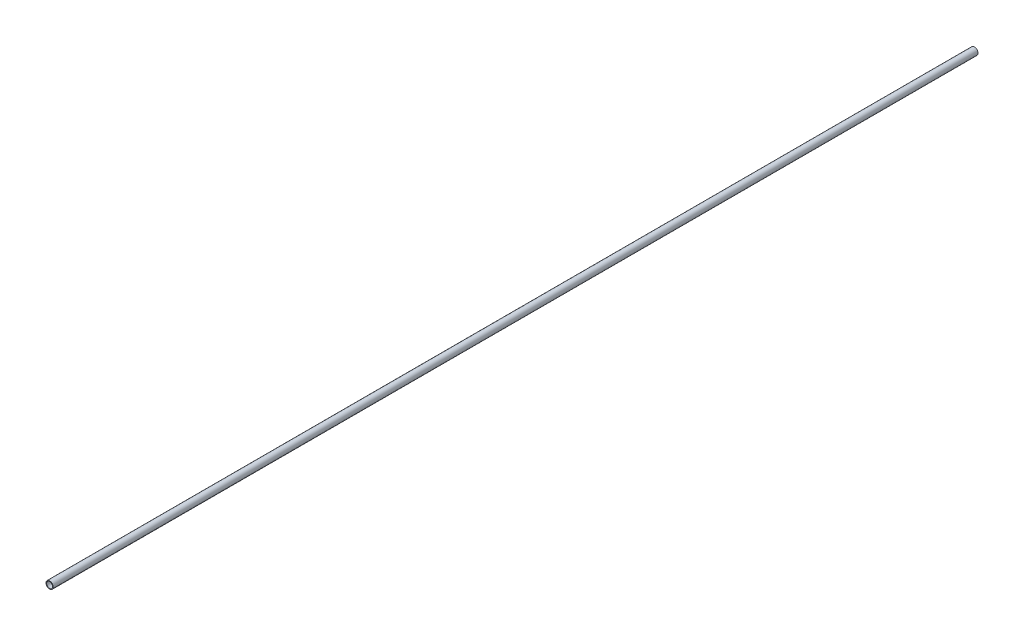
from build123d import *

# Parameters (mm, degrees)
SKETCH1_R           = 17.5
SKETCH1_R_2         = 14.5
BOSS_EXTRUDE1_DEPTH = 4500


with BuildPart() as part:
    # Sketch1 → Boss-Extrude1 (new body)
    with BuildSketch(Plane.XY):
        Circle(SKETCH1_R)
        Circle(SKETCH1_R_2, mode=Mode.SUBTRACT)
    extrude(amount=BOSS_EXTRUDE1_DEPTH)


solid = part.part
